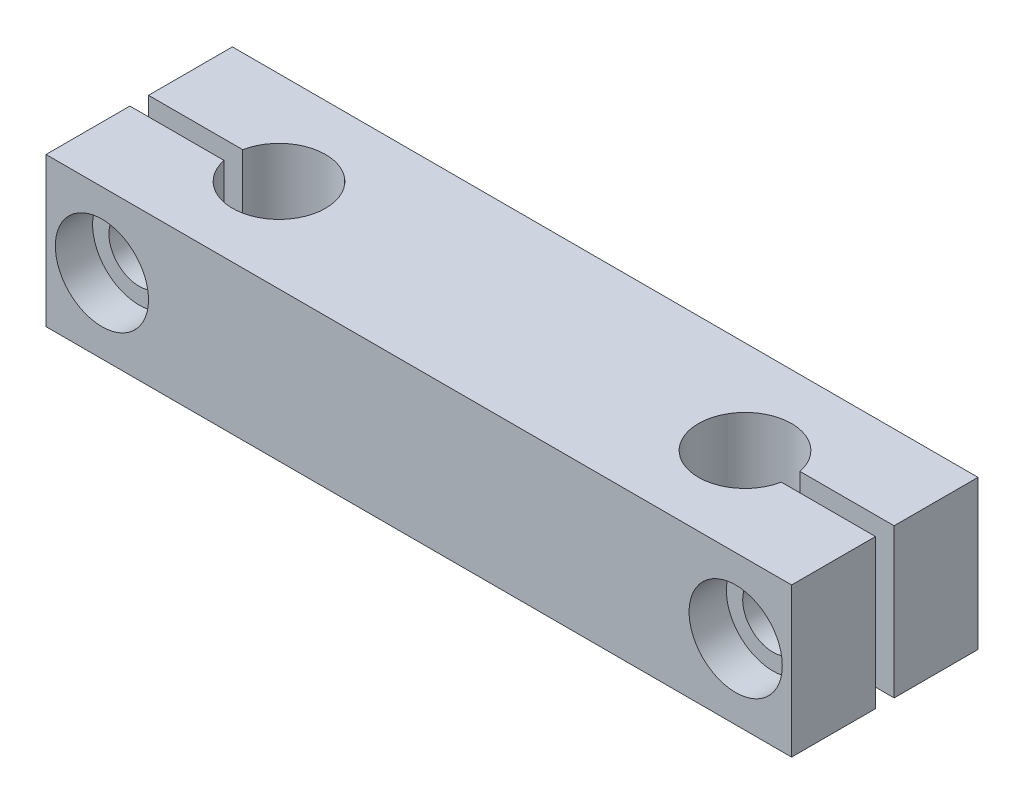
SolidWorks part; units mm, degrees
ref_plane "Front Plane" through (0, 0, 0) normal (0, 0, 1) x (1, 0, 0)
ref_plane "Top Plane" through (0, 0, 0) normal (0, 1, 0) x (1, 0, 0)
ref_plane "Right Plane" through (0, 0, 0) normal (1, 0, 0) x (0, 0, -1)
sketch "Sketch1" plane through (0, 0, 0) normal (0, 0, 1) x (1, 0, 0)
  line L1 (0, 0) -> (-80, 0)
  line L2 (0, 0) -> (0, 16)
  line L3 (0, 16) -> (-80, 16)
  line L4 (-80, 0) -> (-80, 16)
  dimension "D1" = 16
  dimension "D2" = 80
extrude "Boss-Extrude1" add sketch "Sketch1" along normal blind 20
sketch "Sketch2" plane through (0, 0, 0) normal (0, -1, 0) x (1, 0, 0)
  line L0 (0, 20) -> (0, 0) construction
  line L1 (-80, 20) -> (0, 20) construction
  line L3 (-80, 20) -> (-80, 0) construction
  circle A0 centre (-15, 10) radius 5
  circle A1 centre (-65, 10) radius 5
  dimension "D1" = 10
  dimension "D2" = 15
  dimension "D3" = 10
  dimension "D4" = 10
  dimension "D5" = 15
  dimension "D6" = 10
extrude "Cut-Extrude1" cut sketch "Sketch2" against normal blind 20
sketch "Sketch3" plane through (0, 0, 0) normal (0, -1, 0) x (1, 0, 0)
  line L0 (-10, 10) -> (1.4933, 10) construction
  line L1 (-10.945, 9) -> (1.4933, 9)
  line L2 (-10.945, 11) -> (1.4933, 11)
  line L3 (-10, 9) -> (1.4933, 9) construction
  line L4 (-10, 11) -> (1.4933, 11) construction
  line L5 (-10.945, 11) -> (-10.945, 9)
  line L6 (1.4933, 11) -> (1.4933, 9)
  line L7 (-40, 20) -> (-40, -8.0222) construction
  line L8 (-80, 20) -> (0, 20) construction
  line L9 (-70, 10) -> (-81.4933, 10) construction
  line L10 (-81.4933, 11) -> (-81.4933, 9)
  line L11 (-69.055, 11) -> (-69.055, 9)
  line L12 (-69.055, 11) -> (-81.4933, 11)
  line L13 (-69.055, 9) -> (-81.4933, 9)
  circle A0 centre (-15, 10) radius 5 construction
  dimension "D1" = 1
  dimension "D2" = 1
extrude "Cut-Extrude2" cut sketch "Sketch3" against normal blind 30
hole_wizard "M6 Tapped Hole1" positions "Sketch5" profile "Sketch4" tap size "M6" standard "Gb"
sketch "Sketch5" plane through (0, 0, 9) normal (0, 0, 1) x (1, 0, 0)
  line L0 (0, 16) -> (-80, 16) construction
  line L1 (0, 0) -> (0, 16) construction
  line L2 (-80, 16) -> (-80, 0) construction
  point P0 (-6, 8)
  point P2 (-74, 8)
  dimension "D1" = 8
  dimension "D2" = 8
  dimension "D3" = 6
  dimension "D4" = 6
sketch "Sketch4" plane through (-6, 8, 9) normal (1, 0, 0) x (0, -1, 0)
  line L0 (0, 0) -> (0, 18.5022)
  line L1 (0, 18.5022) -> (2.5, 17)
  line L2 (2.5, 17) -> (2.5, 0)
  line L5 (2.5, 0) -> (0, 0)
  line L10 (0, 18.5022) -> (-2.5, 17) construction
  line L11 (0, -6.35) -> (0, 107.95) construction
  dimension "螺纹孔钻头直径" = 5
  dimension "螺纹孔钻头深度" = 17
  dimension "导头角度" = 118
cosmetic thread "CosmeticThread 1" parameters "D1"=9, "D2"=6
cosmetic thread "CosmeticThread 2" parameters "D1"=9, "D2"=6
sketch "Sketch7" plane through (0, 0, 11) normal (0, 0, -1) x (-1, 0, 0)
  circle A0 centre (74, 8) radius 3.25
  circle A1 centre (6, 8) radius 3.25
  dimension "D1" = 6.5
  dimension "D2" = 6.5
extrude "Cut-Extrude3" cut sketch "Sketch7" against normal blind 30
sketch "Sketch8" plane through (0, 0, 20) normal (0, 0, 1) x (1, 0, 0)
  circle A0 centre (-6, 8) radius 5
  circle A1 centre (-74, 8) radius 5
  dimension "D1" = 10
  dimension "D2" = 10
extrude "Cut-Extrude7" cut sketch "Sketch8" against normal blind 4
